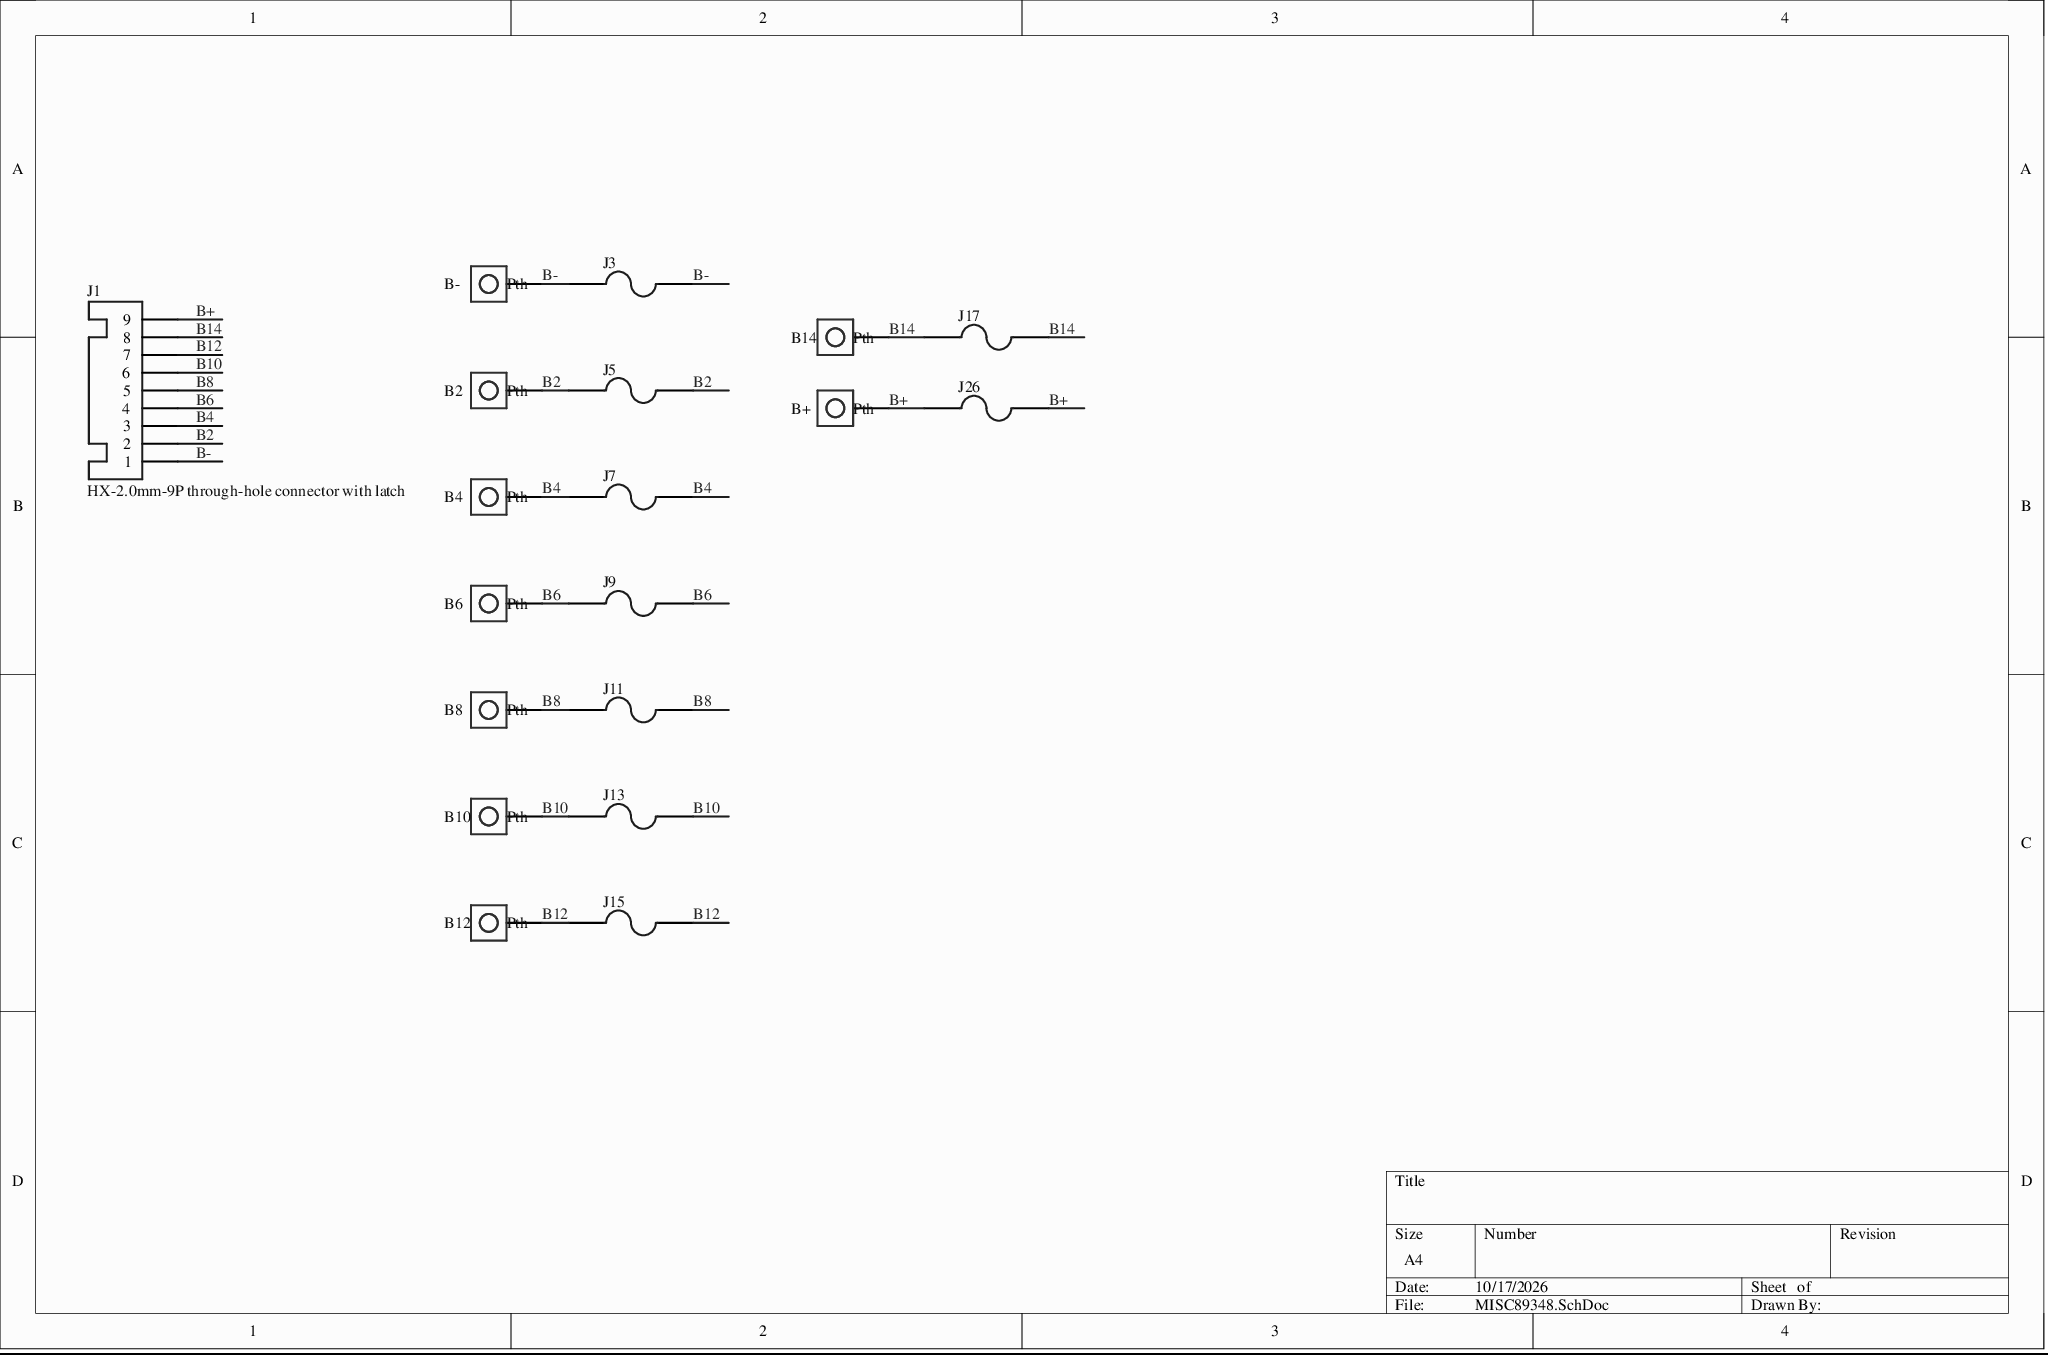
[diagram p0: MISC89348.SchDoc]
# Altium project MISC89348.PrjPcb
1 sheet, 19 parts. Net scope: global (net labels, ports and power ports of the same name join across sheets).
Board file: MISC89348.PcbDoc

## Sheet MISC89348.SchDoc
size A4; SheetNumber: 1; SheetTotal: 1

### Parts
B2  Pth  [55*10*1MM]
B4  Pth  [55*10*1MM]
B6  Pth  [55*10*1MM]
B8  Pth  [161.5*10*1MM]
B10  Pth  [55*10*1MM]
B12  Pth  [55*10*1MM]
B14  Pth  [55*10*1MM]
B+  Pth  [55*10*1MM]
B-  Pth  [55*10*1MM]
J1  HX-2.0mm-9P through-hole connector with latch  [HX2.0-9P]
J3  FPC  [异形电阻]  (value not drawn)
J5  FPC  [异形电阻]  (value not drawn)
J7  FPC  [异形电阻]  (value not drawn)
J9  FPC  [异形电阻]  (value not drawn)
J11  FPC  [异形电阻]  (value not drawn)
J13  FPC  [异形电阻]  (value not drawn)
J15  FPC  [异形电阻]  (value not drawn)
J17  FPC  [异形电阻]  (value not drawn)
J26  FPC  [异形电阻]  (value not drawn)

### Nets
B2: B2.1 J1.2 J5.1 J5.2
B4: B4.1 J1.3 J7.1 J7.2
B6: B6.1 J1.4 J9.1 J9.2
B8: B8.1 J1.5 J11.1 J11.2
B10: B10.1 J1.6 J13.1 J13.2
B12: B12.1 J1.7 J15.1 J15.2
B14: B14.1 J1.8 J17.1 J17.2
B+: B+.1 J1.9 J26.1 J26.2
B-: B-.1 J1.1 J3.1 J3.2

### Library data of the parts
B2 B4 B6 B8 B10 B12 B14 B+ B- = Pth: Through-hole pad
J1 = HX-2.54mm-9P直插带扣: HX-2.54mm-9P through-hole connector with latch